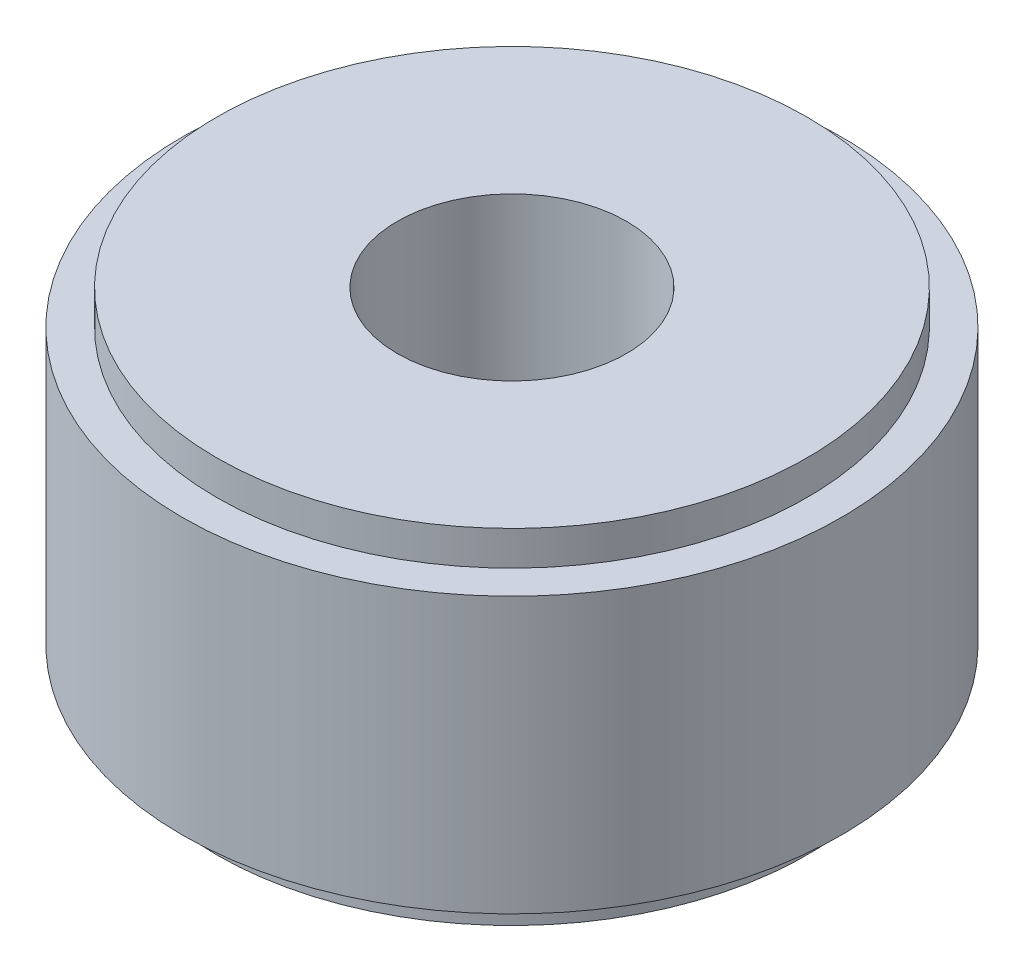
from build123d import *


with BuildPart() as part:
    # 草图1 → 旋转1 (revolve)
    with BuildSketch(Plane.XY, mode=Mode.PRIVATE) as revolve_1_sk:
        Polygon((20, 9.76740105), (20, -50.23259895), (51.5, -50.23259895), (51.5, -44.23259895), (57.5, -44.23259895), (57.5, 3.76740105), (51.5, 3.76740105), (51.5, 9.76740105), align=None)
    revolve(revolve_1_sk.sketch.rotate(Axis((0, 27.589183228, 0), (0, -1, 0)), 90), axis=Axis((0, 27.589183228, 0), (0, -1, 0)))


solid = part.part
